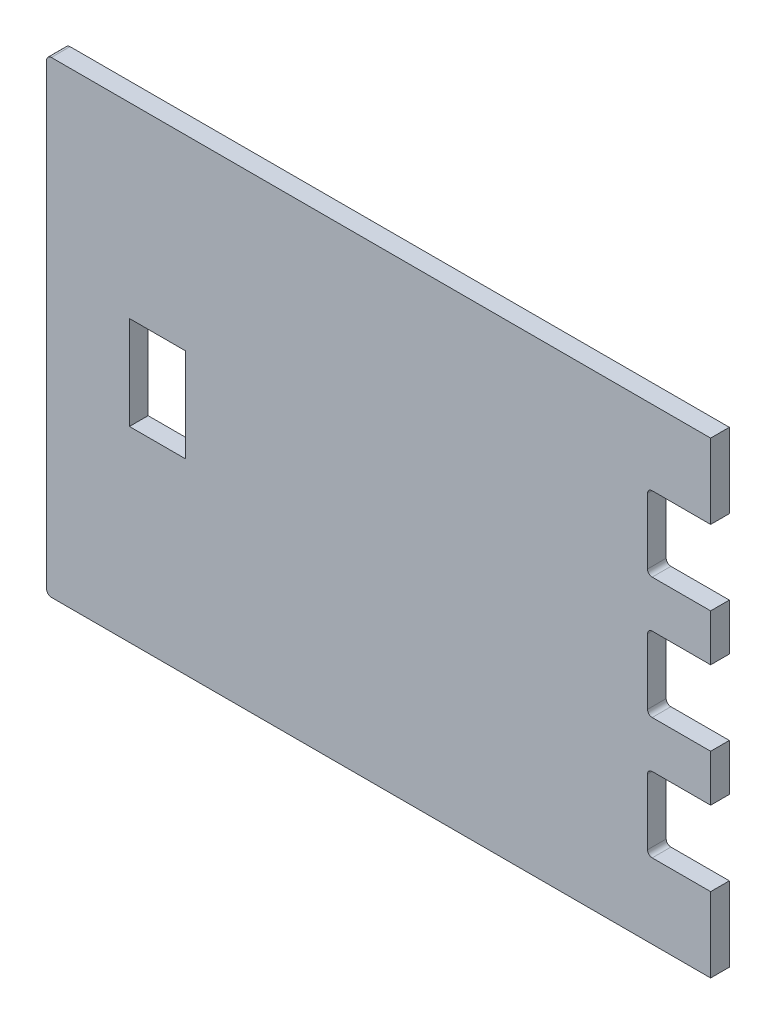
from build123d import *

# Parameters (mm, degrees)
SKETCH1_W           = 120
SKETCH1_H           = 200
BOSS_EXTRUDE1_DEPTH = 40
FILLET1_R           = 10


with BuildPart() as part:
    # Sketch1 → Boss-Extrude1 (new body)
    with BuildSketch(Plane.XY):
        with BuildLine():
            Line((1420, 840), (1295, 840))
            ThreePointArc((1295, 840), (1287.928932188, 837.071067812), (1285, 830))
            Line((1285, 830), (1285, 690))
            ThreePointArc((1285, 690), (1287.928932188, 682.928932188), (1295, 680))
            Line((1295, 680), (1420, 680))
            Line((1420, 680), (1420, 580))
            Line((1420, 580), (1295, 580))
            ThreePointArc((1295, 580), (1287.928932188, 577.071067812), (1285, 570))
            Line((1285, 570), (1285, 430))
            ThreePointArc((1285, 430), (1287.928932188, 422.928932188), (1295, 420))
            Line((1295, 420), (1420, 420))
            Line((1420, 420), (1420, 320))
            Line((1420, 320), (1295, 320))
            ThreePointArc((1295, 320), (1287.928932188, 317.071067812), (1285, 310))
            Line((1285, 310), (1285, 170))
            ThreePointArc((1285, 170), (1287.928932188, 162.928932188), (1295, 160))
            Line((1295, 160), (1420, 160))
            Line((1420, 160), (1420, 0))
            Line((1420, 0), (0, 0))
            Line((0, 0), (0, 1000))
            Line((0, 1000), (1420, 1000))
            Line((1420, 1000), (1420, 840))
        make_face()
        with Locations((237, 500)):
            Rectangle(SKETCH1_W, SKETCH1_H, mode=Mode.SUBTRACT)
    extrude(amount=BOSS_EXTRUDE1_DEPTH)

    # Fillet1
    fillet1_edges = [part.edges().sort_by_distance(p)[0] for p in [
        (0, 1000, 20),
        (0, 0, 20),
    ]]
    fillet(fillet1_edges, radius=FILLET1_R)


solid = part.part
